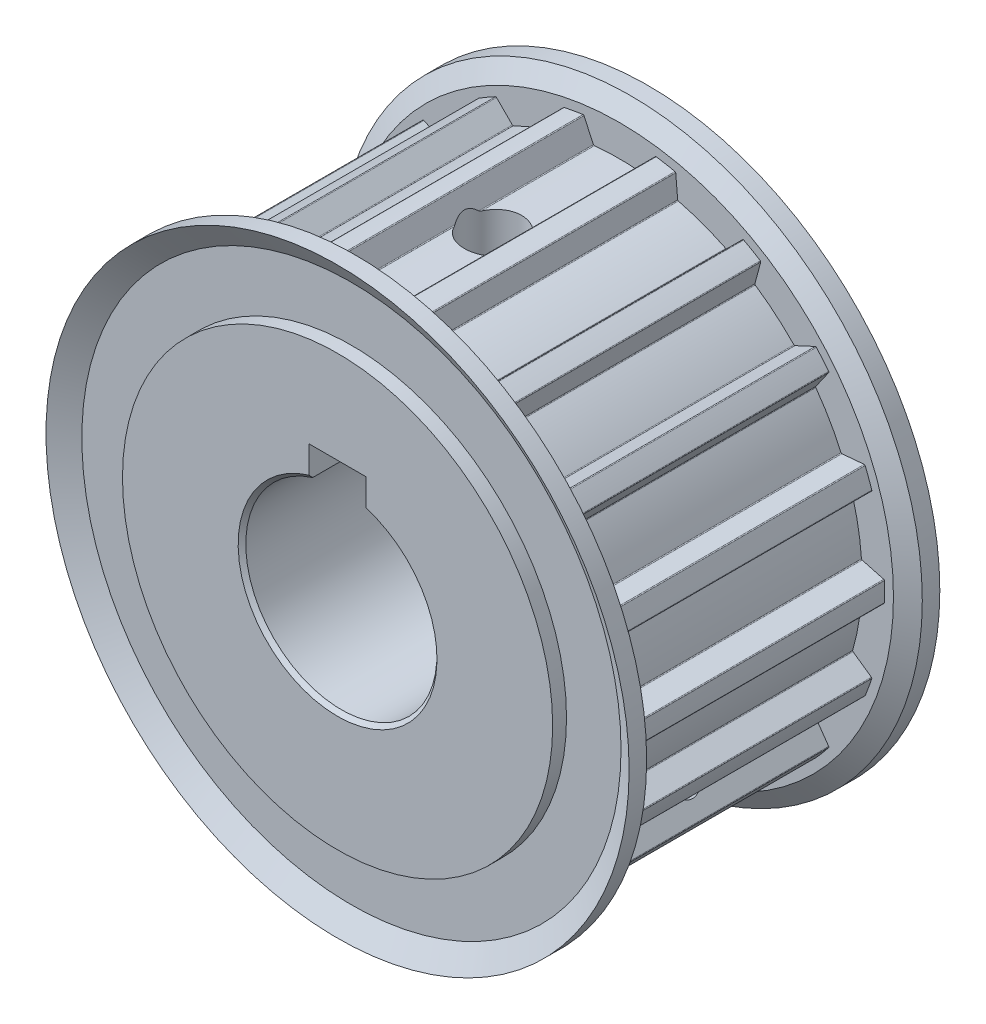
SolidWorks part; units mm, degrees
ref_plane "Front Plane" through (0, 0, 0) normal (0, 0, 1) x (1, 0, 0)
ref_plane "Top Plane" through (0, 0, 0) normal (0, 1, 0) x (1, 0, 0)
ref_plane "Right Plane" through (0, 0, 0) normal (1, 0, 0) x (0, 0, -1)
sketch "Sketch1" plane through (0, 0, 0) normal (1, 0, 0) x (0, 0, -1)
  line L0 (-16.25, 0) -> (16.25, 0) construction
  line L1 (16.25, 0) -> (16.25, 22.5)
  line L2 (16.25, 22.5) -> (14.8, 22.5)
  line L3 (14.8, 22.5) -> (14.8, 28.2019)
  line L4 (14.8, 28.2019) -> (16.25, 30.5)
  line L5 (16.25, 30.5) -> (14.4173, 30.5)
  line L6 (14.4173, 30.5) -> (13.25, 28.65)
  line L7 (13.25, 28.65) -> (13.25, 27.725)
  line L8 (0, 0) -> (0, 30.5) construction
  line L9 (-31.75, 0) -> (-49.75, 0) construction
  line L10 (-31.75, 0) -> (-16.25, 0) construction
  line L11 (-16.25, 17.5) -> (-31.75, 17.5)
  line L12 (-31.75, 17.5) -> (-31.75, 0)
  line L13 (-26.75, 17.5) -> (-26.75, 0) construction
  point P10 (13.25, 27.725)
  dimension "D1" = 3
  dimension "W" = 32.5
  dimension "F" = 61
  dimension "D2" = 1.55
  dimension "E" = 45
  dimension "D3" = 1.55
  dimension "PD" = 57.3
  dimension "OD" = 55.45
  dimension "D4" = 5
  dimension "CS" = 18
  dimension "L" = 48
  dimension "D" = 35
sketch "Sketch2" plane through (0, 0, 0) normal (0, 0, 1) x (1, 0, 0)
  line L0 (0, 27.725) -> (0, -27.725) construction
  line L1 (0, 25.365) -> (0, 27.725) construction
  line L3 (2.7352, 25.285) -> (3.7227, 27.4028)
  line L4 (-2.705, 25.2204) -> (0, 0) construction
  line L5 (0, 0) -> (0, 25.365) construction
  line L6 (0, 0) -> (4.8144, 27.3038) construction
  circle A2 centre (0, 0) radius 25.365 construction
  circle A9 centre (0, 0) radius 27.725 construction
  arc A12 (2.6342, 25.2279) -> (-2.705, 25.2204) centre (0, 0) ccw
  arc A13 (5.8677, 27.097) -> (3.8271, 27.4596) centre (0, 0) ccw
  arc A14 (2.6342, 25.2279) -> (2.7352, 25.285) centre (2.6445, 25.3273) ccw
  arc A15 (3.7227, 27.4028) -> (3.8271, 27.4596) centre (3.8133, 27.3605) cw
  point P6 (0, 25.365)
  point P17 (2.705, 25.2204)
  point P20 (3.7539, 27.4697)
  point P29 (0, 27.725)
  dimension "D1" = 2.36
  dimension "D5" = 0.1
  dimension "D6" = 10
  dimension "D2" = 5.41
  dimension "D7" = 0.1
  dimension "D3" = 25
sketch "Sketch3" plane through (0, 0, 0) normal (1, 0, 0) x (0, 0, -1)
  line L0 (16.25, 0) -> (16.25, 22.5) construction
  line L1 (16.25, 22.5) -> (14.8, 22.5) construction
  line L2 (14.8, 22.5) -> (14.8, 28.2019) construction
  line L3 (14.8, 28.2019) -> (16.25, 30.5) construction
  line L4 (16.25, 30.5) -> (14.4173, 30.5) construction
  line L5 (14.4173, 30.5) -> (13.25, 28.65) construction
  line L7 (16.25, 0) -> (16.25, 22.5)
  line L8 (16.25, 22.5) -> (14.8, 22.5)
  line L9 (14.8, 22.5) -> (14.8, 28.2019)
  line L10 (14.8, 28.2019) -> (16.25, 30.5)
  line L11 (16.25, 30.5) -> (14.4173, 30.5)
  line L12 (14.4173, 30.5) -> (13.25, 28.65)
  line L13 (13.25, 28.65) -> (13.25, 25.365)
  line L15 (13.25, 25.365) -> (-13.25, 25.365)
  line L16 (0, 0) -> (0, 30.5) construction
  line L17 (0, 0) -> (0, 30.5) construction
  line L18 (-13.25, 28.65) -> (-13.25, 25.365)
  line L19 (-14.4173, 30.5) -> (-13.25, 28.65)
  line L20 (-16.25, 30.5) -> (-14.4173, 30.5)
  line L21 (-14.8, 28.2019) -> (-16.25, 30.5)
  line L22 (-14.8, 22.5) -> (-14.8, 28.2019)
  line L23 (-16.25, 22.5) -> (-14.8, 22.5)
  line L24 (-16.25, 0) -> (-16.25, 22.5)
  line L25 (-16.25, 0) -> (16.25, 0)
  point P14 (0, 25.365)
revolve "Revolve1" add sketch "Sketch3" angle 360 about L0
sketch "Sketch4" plane through (0, 0, 0) normal (0, 0, 1) x (1, 0, 0)
  line L1 (0, 0) -> (4.8144, 27.3038) construction
  line L2 (0, 0) -> (4.8144, 27.3038) construction
  line L3 (2.7352, 25.285) -> (3.7227, 27.4028) construction
  line L4 (2.7352, 25.285) -> (3.7227, 27.4028)
  line L5 (6.0778, 24.6957) -> (5.8741, 27.0234)
  arc A1 (2.6342, 25.2279) -> (2.7352, 25.285) centre (2.6445, 25.3273) ccw construction
  arc A3 (3.8271, 27.4596) -> (3.7227, 27.4028) centre (3.8133, 27.3605) ccw construction
  arc A4 (5.8677, 27.097) -> (3.8271, 27.4596) centre (0, 0) ccw construction
  arc A5 (2.6342, 25.2279) -> (2.7352, 25.285) centre (2.6445, 25.3273) ccw
  arc A6 (3.8271, 27.4596) -> (3.7227, 27.4028) centre (3.8133, 27.3605) ccw
  arc A7 (5.7954, 27.1125) -> (3.8271, 27.4596) centre (0, 0) ccw
  circle A8 centre (0, 0) radius 25.365 construction
  arc A10 (6.1531, 24.6074) -> (2.6342, 25.2279) centre (0, 0) ccw
  arc A11 (6.1531, 24.6074) -> (6.0778, 24.6957) centre (6.1774, 24.7044) cw
  arc A12 (5.7954, 27.1125) -> (5.8741, 27.0234) centre (5.7745, 27.0147) cw
extrude "Boss-Extrude1" add sketch "Sketch4" along normal mid plane 26.5
pattern_circular "CirPattern1" count 18 over 360 about axis through (0, 0, 0) along (0, 0, 1) of "Boss-Extrude1"
sketch "Sketch14" plane through (0, 0, 0) normal (1, 0, 0) x (0, 0, -1)
  line L0 (-16.25, 30.5) -> (-16.25, -30.5) construction
  line L1 (-31.75, 17.5) -> (-16.25, 17.5)
  line L2 (-31.75, 17.5) -> (-31.75, 0)
  line L3 (-31.75, 0) -> (-16.25, 0)
  line L4 (-16.25, 17.5) -> (-16.25, 0)
revolve "Revolve2" [suppressed] add sketch "Sketch14" angle 360 about L3
sketch "Sketch H" plane through (0, 0, 0) normal (1, 0, 0) x (0, 0, -1)
  line L0 (16.25, 0) -> (16.25, 22.5) construction
  line L1 (-16.25, 0) -> (16.25, 0) construction
  line L2 (-16.25, 0) -> (16.25, 0) construction
  point P0 (16.25, 0.5)
  dimension "dH" = 1
sketch "Sketch6" [suppressed] plane through (0, 0, 0) normal (0, 0, 1) x (1, 0, 0)
  circle A0 centre (0, 0) radius 17.5
extrude "Cut-Extrude1" [suppressed] cut sketch "Sketch6" against normal through all and the other way through all
chamfer "Chamfer1" [suppressed] distance 0.21 angle 45
sketch "Sketch P" plane through (0, 0, 0) normal (0, 0, 1) x (1, 0, 0)
  line L0 (0, 0) -> (0, 30.5) construction
  line L1 (0, 0) -> (0, 30.5) construction
  circle A0 centre (0, 0) radius 0.5
  point P3 (0.25, 0.433)
  dimension "dP" = 1
  dimension "MP" = 0.5
sketch "Sketch19" [suppressed] plane through (0, 0, 0) normal (0, 0, 1) x (1, 0, 0)
  circle A0 centre (0, 0) radius 2.5 construction
  circle A1 centre (0, 0) radius 2.5
extrude "Cut-Extrude5" [suppressed] cut sketch "Sketch19" against normal through all and the other way through all
chamfer "Chamfer6" [suppressed] distance 0.05 angle 45
sketch "Sketch20" [suppressed] plane through (0, 0, 0) normal (0, 1, 0) x (1, 0, 0)
  circle A0 centre (0, 0) radius 1.5
  point P4 (1.5, 0)
extrude "Cut-Extrude6" cut sketch "Sketch20" along normal through all
cosmetic thread "Cosmetic Thread3" [suppressed] parameters "D2"=0.6
ref_plane "Plane2" [suppressed] through (0, 0, 0) normal (-0.866, 0.5, 0) x (-0.5, -0.866, 0)
sketch "Sketch21" [suppressed] plane through (0, 0, 0) normal (-0.866, 0.5, 0) x (-0.5, -0.866, 0)
  circle A0 centre (0, 0) radius 1.5
  dimension "D1" = 0.5
extrude "Cut-Extrude7" cut sketch "Sketch21" against normal through all
cosmetic thread "Cosmetic Thread4" [suppressed] parameters "D2"=0.6
chamfer "Chamfer7" [suppressed] distance 0.035 angle 45
sketch "Sketch N" plane through (0, 0, 0) normal (0, 0, 1) x (1, 0, 0)
  line L0 (-3, 9.5394) -> (-3, 12.8)
  line L1 (-3, 12.8) -> (3, 12.8)
  line L2 (3, 12.8) -> (3, 9.5394)
  line L3 (0, 0) -> (0, 30.5) construction
  line L4 (0, 0) -> (0, 30.5) construction
  arc A0 (-3, 9.5394) -> (3, 9.5394) centre (0, 0) ccw
  point P1 (0, 10)
  point P8 (3, 12.8)
  dimension "dN" = 20
  dimension "bN" = 6
  dimension "tN" = 2.8
  dimension "MN" = 6
sketch "Sketch9" plane through (0, 0, 0) normal (0, 0, 1) x (1, 0, 0)
  line L0 (-3, 9.5394) -> (-3, 12.8) construction
  line L1 (-3, 12.8) -> (3, 12.8) construction
  line L2 (3, 12.8) -> (3, 9.5394) construction
  line L3 (-3, 9.5394) -> (-3, 12.8)
  line L4 (-3, 12.8) -> (3, 12.8)
  line L5 (3, 12.8) -> (3, 9.5394)
  arc A0 (-3, 9.5394) -> (3, 9.5394) centre (0, 0) ccw construction
  arc A1 (-3, 9.5394) -> (3, 9.5394) centre (0, 0) ccw
extrude "Cut-Extrude2" cut sketch "Sketch9" against normal through all and the other way through all
chamfer "Chamfer2" distance 0.4 angle 45 2 edges at (0, -10, -16.25) (0, -10, 16.25)
sketch "Sketch15" plane through (0, 0, 0) normal (0, 1, 0) x (1, 0, 0)
  circle A0 centre (0, 0) radius 3
  point P2 (3, 0)
extrude "Cut-Extrude3" cut sketch "Sketch15" along normal through all from vertex at 12.8 starting at point (3, 12.8, 0)
cosmetic thread "Cosmetic Thread1" parameters "D2"=6.1
ref_plane "Plane1" through (0, 0, 0) normal (-0.866, 0.5, 0) x (-0.5, -0.866, 0)
sketch "Sketch16" plane through (0, 0, 0) normal (-0.866, 0.5, 0) x (-0.5, -0.866, 0)
  circle A0 centre (0, 0) radius 3
  dimension "D1" = 6
extrude "Cut-Extrude4" cut sketch "Sketch16" against normal through all
cosmetic thread "Cosmetic Thread2" parameters "D2"=6.1
chamfer "Chamfer5" [suppressed] distance 0.3 angle 45
sketch "Sketch V" plane through (0, 0, 0) normal (1, 0, 0) x (0, 0, -1)
  line L0 (-16.25, 0.5) -> (14.25, 0.5)
  line L1 (14.25, 0.5) -> (14.25, 1.5)
  line L2 (14.25, 1.5) -> (16.25, 1.5)
  line L3 (-16.25, 0) -> (16.25, 0) construction
  line L4 (-16.25, 0) -> (16.25, 0) construction
  dimension "dV" = 1
  dimension "ZV" = 3
  dimension "JV" = 2
sketch "Sketch11" [suppressed] plane through (0, 0, 0) normal (1, 0, 0) x (0, 0, -1)
  line L1 (1.5, 4) -> (1.5, 5) construction
  line L2 (1.5, 5) -> (5.5, 5) construction
  line L3 (-5.5, 4) -> (1.5, 4)
  line L4 (1.5, 4) -> (1.5, 5)
  line L5 (1.5, 5) -> (5.5, 5)
  line L6 (-5.5, 4) -> (-5.5, 0)
  line L7 (-5.5, 0) -> (5.5, 0)
  line L8 (5.5, 0) -> (5.5, 5)
revolve "Cut-Revolve1" [suppressed] cut sketch "Sketch11" angle 360 about L0
chamfer "Chamfer3" [suppressed] distance 0.13 angle 45
sketch "Sketch F" plane through (0, 0, 0) normal (1, 0, 0) x (0, 0, -1)
  line L0 (-16.25, 0) -> (16.25, 0) construction
  line L3 (-16.25, 0) -> (16.25, 0) construction
  line L4 (-16.25, 0) -> (-16.25, 5)
  line L5 (-16.25, 30.5) -> (-16.25, -30.5) construction
  line L8 (-16.25, 5) -> (-12.25, 5)
  line L9 (-12.25, 5) -> (-12.25, 4)
  line L10 (-12.25, 4) -> (16.25, 4)
  line L11 (16.25, 4) -> (16.25, 0)
  dimension "ZF" = 10
  dimension "dF" = 8
  dimension "JF" = 4
sketch "Sketch22" [suppressed] plane through (0, 0, 0) normal (1, 0, 0) x (0, 0, -1)
  line L0 (-11.5, 0) -> (-11.5, 5)
  line L2 (-11.5, 7) -> (-11.5, 0) construction
  line L3 (-11.5, 5) -> (-7.5, 5)
  line L4 (-5, 5) -> (-1, 5) construction
  line L6 (-7.5, 5) -> (-7.5, 4)
  line L9 (5, 4) -> (5, 0)
  line L10 (5, 0) -> (-11.5, 0)
  line L11 (-7.5, 4) -> (5, 4)
revolve "Cut-Revolve3" [suppressed] cut sketch "Sketch22" angle 360 about L10
chamfer "Chamfer8" [suppressed] distance 0.18 angle 45
sketch "Sketch Y" plane through (0, 0, 0) normal (1, 0, 0) x (0, 0, -1)
  line L2 (-16.25, 0) -> (16.25, 0) construction
  line L3 (-16.25, 0) -> (16.25, 0) construction
  line L4 (-16.25, 0.05) -> (-13.25, 0.05)
  line L5 (-13.25, 0.05) -> (-13.25, 1.5)
  line L6 (-13.25, 1.5) -> (13.25, 1.5)
  line L7 (13.25, 1.5) -> (13.25, 0.05)
  line L8 (13.25, 0.05) -> (16.25, 0.05)
  dimension "dY" = 3
  dimension "QY" = 0.1
  dimension "RY" = 0.1
  dimension "SY" = 3
  dimension "TY" = 3
sketch "Sketch13" [suppressed] plane through (0, 0, 0) normal (1, 0, 0) x (0, 0, -1)
  line L0 (-5.5, 4) -> (-2.5, 4) construction
  line L1 (-2.5, 4) -> (-2.5, 2.5) construction
  line L2 (-2.5, 2.5) -> (2.5, 2.5) construction
  line L3 (2.5, 2.5) -> (2.5, 4.5) construction
  line L4 (2.5, 4.5) -> (5.5, 4.5) construction
  line L5 (-5.5, 4) -> (-2.5, 4)
  line L6 (-2.5, 4) -> (-2.5, 2.5)
  line L7 (-2.5, 2.5) -> (2.5, 2.5)
  line L8 (2.5, 2.5) -> (2.5, 4.5)
  line L9 (2.5, 4.5) -> (5.5, 4.5)
  line L10 (-5.5, 4) -> (-5.5, 0)
  line L11 (-5.5, 0) -> (5.5, 0)
  line L12 (5.5, 0) -> (5.5, 4.5)
revolve "Cut-Revolve2" [suppressed] cut sketch "Sketch13" angle 360 about L0
chamfer "Chamfer4" [suppressed] distance 0.02 angle 45
sketch "Sketch23" [suppressed] plane through (0, 0, 0) normal (0, 0, 1) x (1, 0, 0)
  line L0 (0, 5) -> (0, 0) construction
  line L1 (-2, 6.8) -> (2, 6.8)
  line L2 (-2, 6.8) -> (-2, 4.5826)
  line L4 (2, 6.8) -> (2, 4.5826)
  arc A0 (-2, 4.5826) -> (2, 4.5826) centre (0, 0) ccw
  circle A2 centre (0, 0) radius 5 construction
  dimension "D1" = 10
  dimension "D2" = 4
  dimension "D3" = 1.8
extrude "Cut-Extrude8" [suppressed] cut sketch "Sketch23" against normal through all and the other way through all
chamfer "Chamfer9" [suppressed] distance 0.3 angle 45
sketch "Sketch24" [suppressed] plane through (0, 0, 0) normal (0, 1, 0) x (1, 0, 0)
  circle A0 centre (0, 0) radius 2
  dimension "D1" = 4
extrude "Cut-Extrude9" cut sketch "Sketch24" along normal through all
cosmetic thread "Cosmetic Thread5" [suppressed] parameters "D2"=4.1
pattern_circular "CirPattern2" [suppressed] count 2 over 120
